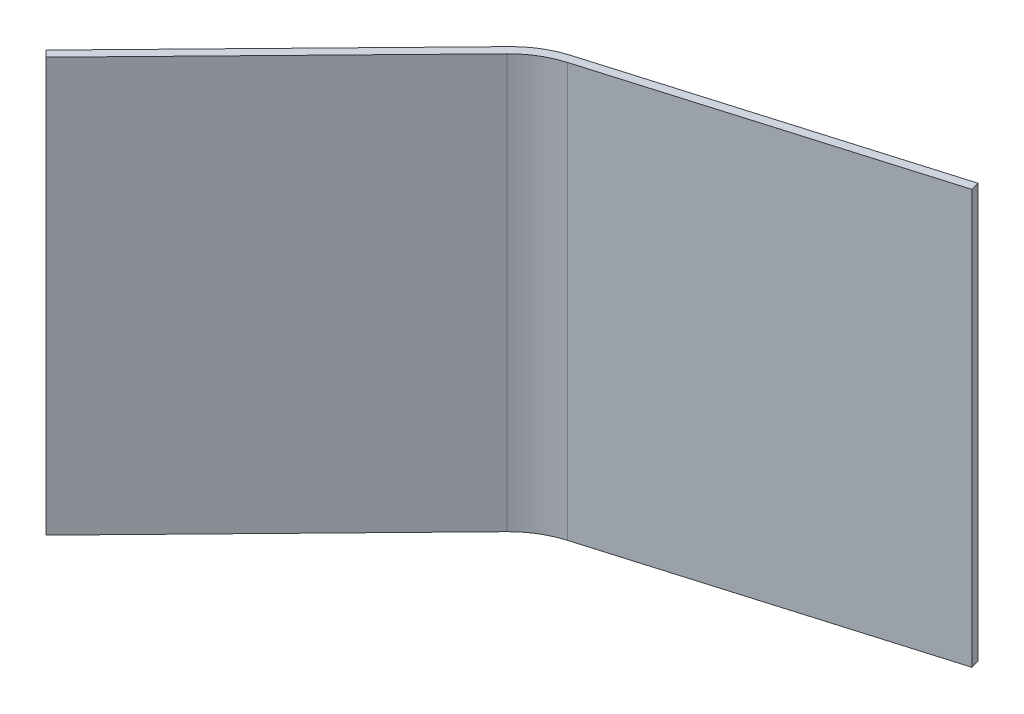
from build123d import *

# Parameters (mm, degrees)
BOSS_EXTRUDE1_DEPTH = 475
FILLET1_R           = 100


with BuildPart() as part:
    # Sketch1 → Boss-Extrude1 (new body)
    with BuildSketch(Plane(origin=(0, 0, 0), x_dir=(1, 0, 0), z_dir=(0, 1, 0))):
        Polygon((0, 0), (279.136209435, 286.501268029), (662.731460294, 399.879764751), (659.896997876, 409.469646022), (273.796619493, 295.350713666), (-7.162531701, 6.978405236), align=None)
    extrude(amount=BOSS_EXTRUDE1_DEPTH)

    # Fillet1
    fillet1_edges = [part.edges().sort_by_distance(p)[0] for p in [
        (273.796619493, 237.5, -295.350713666),
        (279.136209435, 237.5, -286.501268029),
    ]]
    fillet(fillet1_edges, radius=FILLET1_R)


solid = part.part
